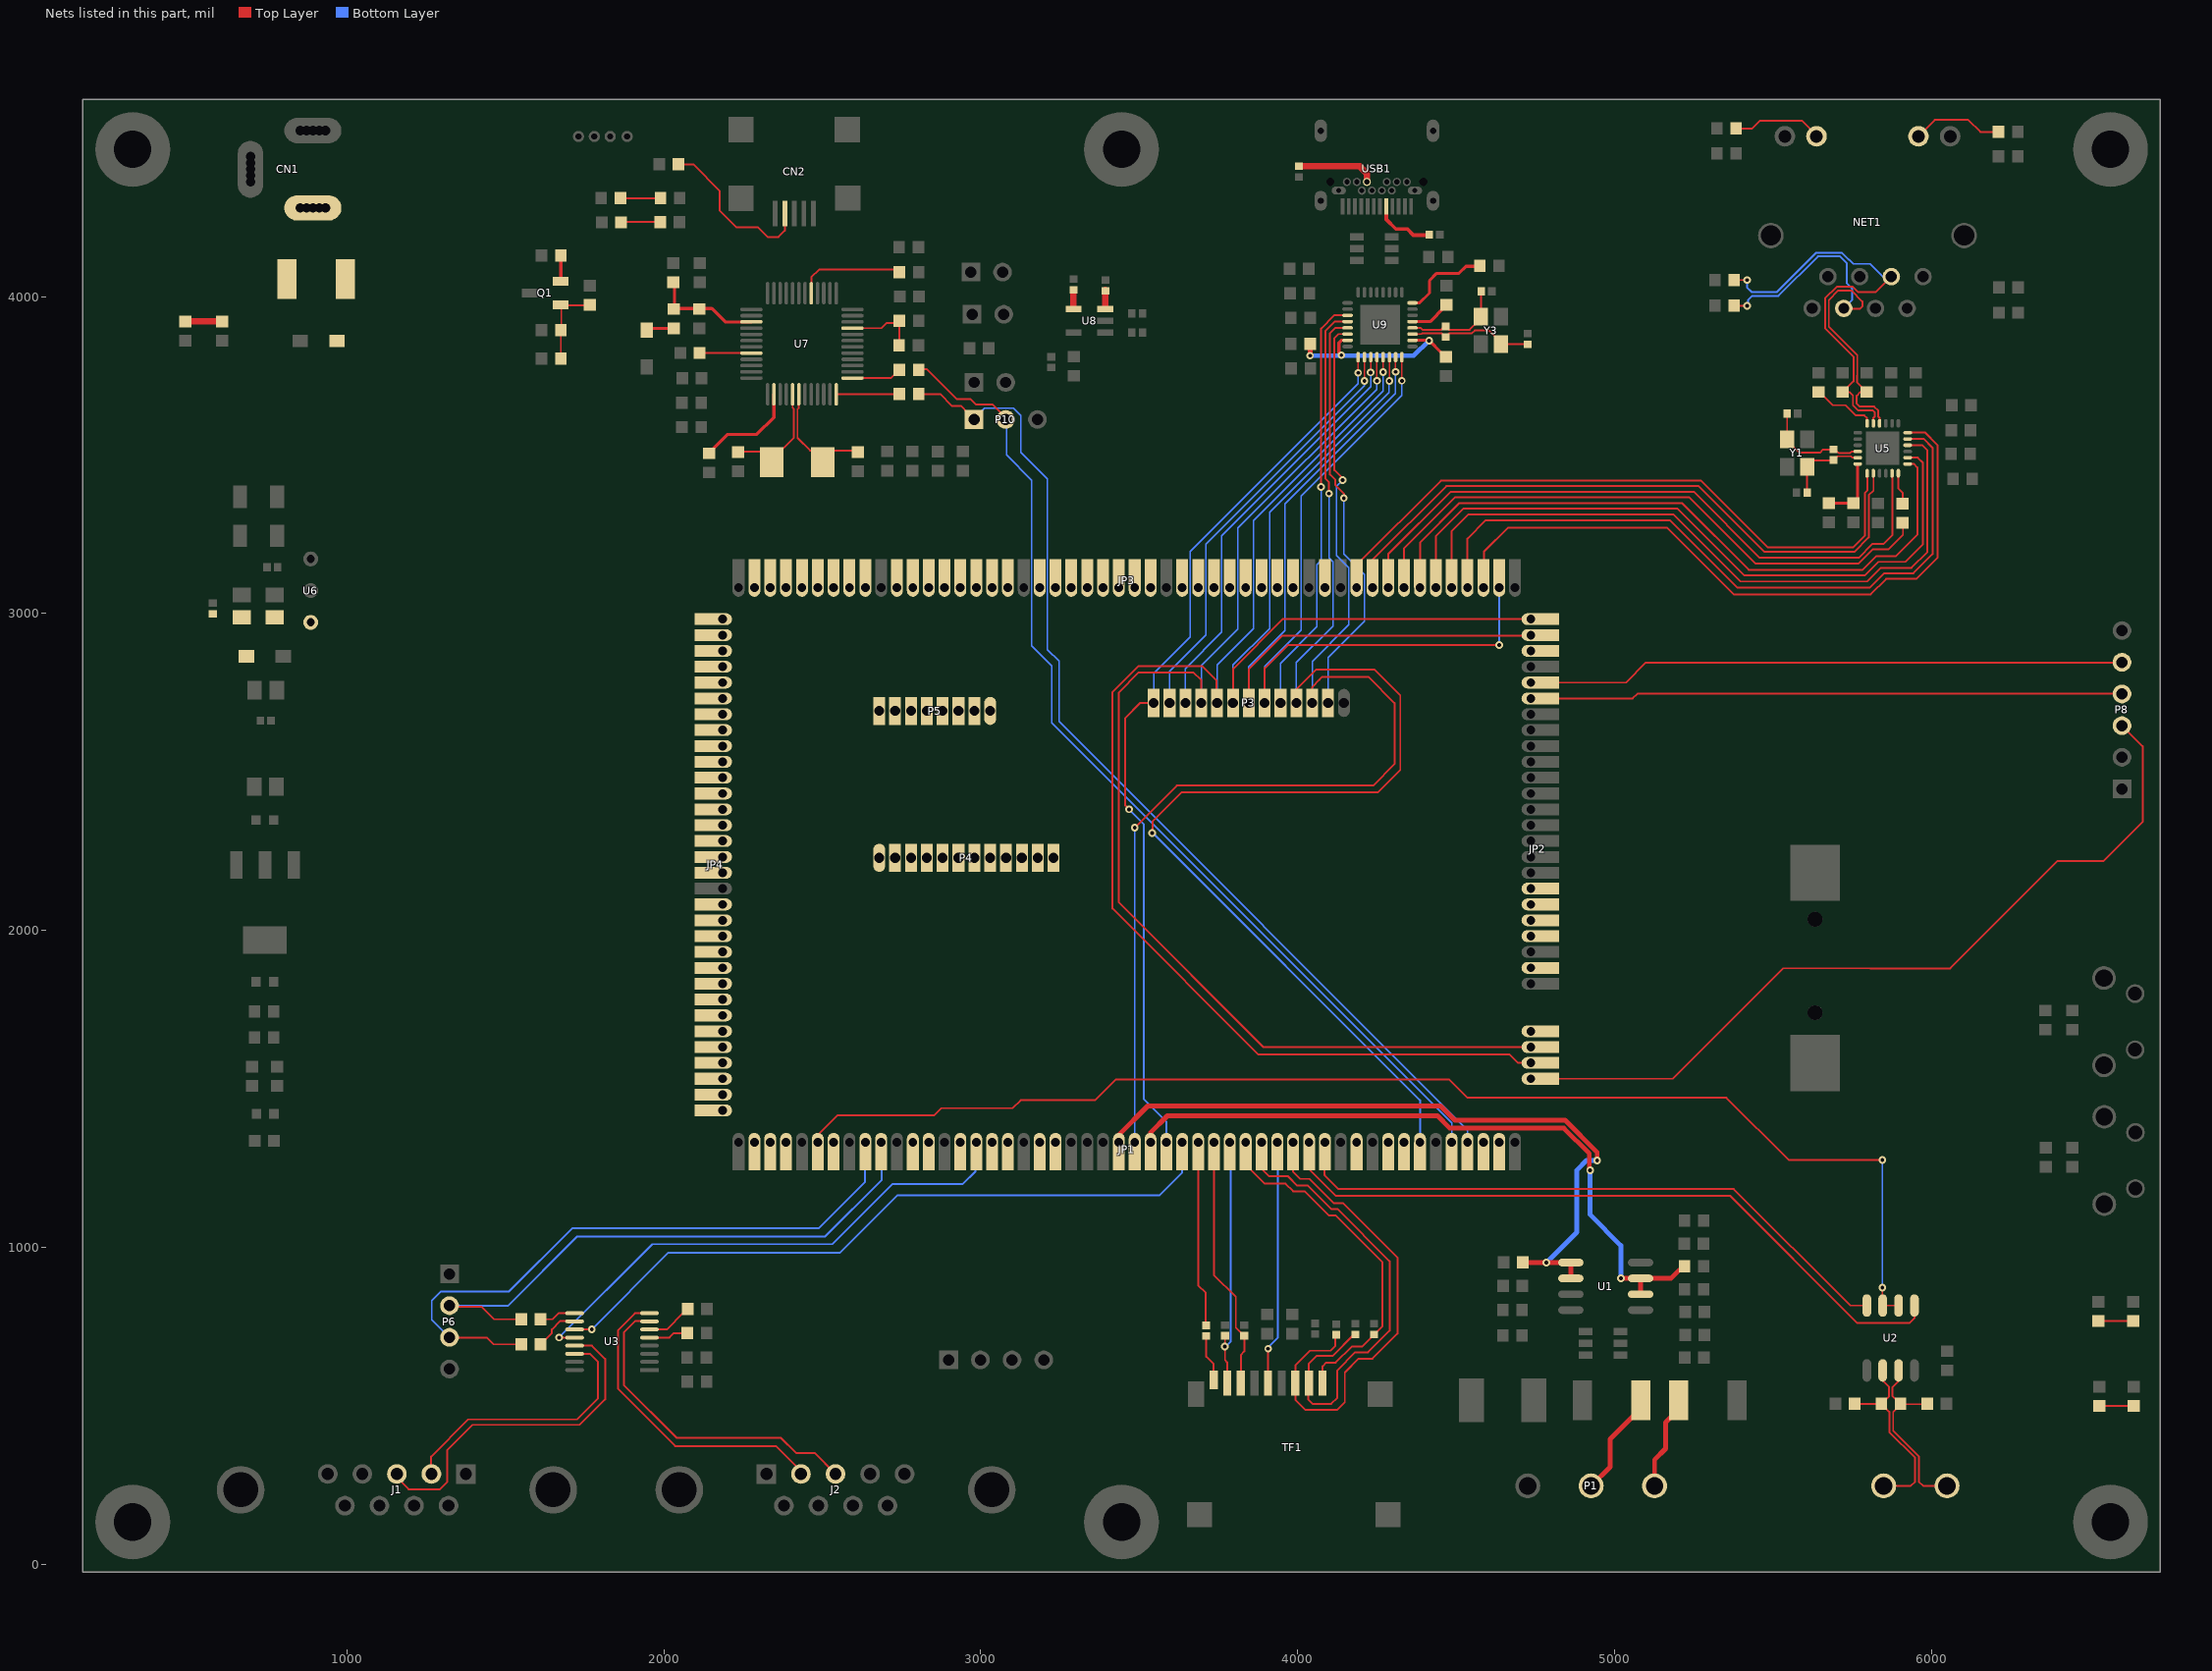
[diagram p0: the nets of this part, all layers, seen from the top]
# Altium PCB MISC105202-15.PcbDoc (part 3 of 4)
Units mil, origin at the board's own origin, x right, y up, seen from the top; angles counter-clockwise.
Board outline 6555.12 x 4645.67 mil, 2 copper layers (Top Layer, Bottom Layer); 182 components, 258 nets, 994 pads, 145 vias.
Unrouted connection lines stored in the file: 1.

## Via types
v1: diameter 24, hole 12, Top Layer to Bottom Layer, 128 vias
v2: diameter 19.68, hole 7.87, Top Layer to Bottom Layer, 9 vias
v3: diameter 50, hole 50, Top Layer to Bottom Layer, 4 vias
v4: diameter 30, hole 15, Top Layer to Bottom Layer, 2 vias
v5: diameter 137.8, hole 137.8, Top Layer to Bottom Layer, 2 vias

## Nets (pads, with @x,y where several pads share a name; then routed paths per layer and width w, separated by ;. In a path a pad name is that pad's centre, name@x,y a point inside that pad or via, vN(x,y) a via of type N, cw(c..) or ccw(c..) an arc to the next point about the centre after c; other vN are vias at no path point) (continued)
NetC9_2: C9.2 U3.5 | length 119.6
  Top Layer w6: U3.5@1955,715.36 2018.36,715.36 2032,729 C9.2@2069,729
NetC11_2: C11.2 U3.6 | length 130
  Top Layer w6: U3.6@1955,740.95 2009.95,740.95 C11.2@2063,794
NetC25_2: C25.2 C26.2 U5.6 | length 202.7
  Top Layer w10: C25.2@5676,3348.31 C26.2@5754,3348.31 C26.2@5754.32,3348.31 ; C26.2@5766,3346 5767,3347 5767,3393 5767,3399 U5.6@5767,3470
NetC27_1: C27.1 R32.2 U5.4 Y1.1 | length 314.9
  Top Layer w6: C27.1@5544.5,3624.5 Y1.1@5544.5,3549.31 5544.5,3545.5 5583,3507 5648,3507 5658,3517 R32.2@5688,3517 ; R32.2@5700,3513 5707,3506 5743,3506 5748.16,3511.16 U5.4@5767.26,3511.16
NetC29_1: C29.1 R32.1 U5.5 Y1.3 | length 214
  Top Layer w6: C29.1@5607.73,3381 Y1.3@5607.73,3452.73 ; Y1.3@5620,3483 5689.73,3483 R32.1@5691,3484.27 ; R32.1@5700,3492 5704,3496 5746,3496 5750.53,3491.47 U5.5@5767.26,3491.47
NetC31_2: C31.2 C32.2 C33.1 D7.1 U6.3
NetC57_2: C57.2 U8.4 | length 60.3
  Top Layer w20: U8.4@3293,3961 3293,3969 C57.2@3293,4021.27
NetC63_1: C63.1 R60.2 U9.27 Y3.3 | length 357.8
  Top Layer w6: U9.27@4362.36,3881.47 4390.47,3881.47 4393,3884 4454,3884 R60.2@4461,3877 ; R60.2@4467,3872.27 4478.73,3884 4550,3884 4559,3893 4604,3893 Y3.3@4628,3869 ; Y3.3@4650.27,3849.27 C63.1@4726,3849.27
NetC64_1: C64.1 R60.1 U9.28 Y3.1 | length 305
  Top Layer w6: U9.28@4362.36,3901.16 4387.84,3901.16 4394,3895 4453,3895 R60.1@4461,3903 ; R60.1@4467,3905.73 4477.73,3895 4543,3895 Y3.1@4570,3922 ; C64.1@4578,4018 4578.5,4017.5 Y3.1@4578.5,3936.31
NetC65_2: C65.2 U9.29 | length 117.9
  Top Layer w10: U9.29@4362.36,3920.84 4417.84,3920.84 C65.2@4462,3965
NetC66_2: C66.2 C67.2 U9.15 U9.26 | length 606.2
  Top Layer w4: C67.2@4044,3852 C67.2@4044.21,3851.79
  Top Layer w10: v1(4039.31,3813.31) v1@4039.31,3819.69 ; v1@4130,3823 4130,3854 4137.79,3861.79 U9.15@4157.64,3861.79 ; U9.26@4362.36,3861.79 4414.21,3861.79 v1(4415,3861) C66.2@4454,3822
  Top Layer w15: C67.2@4039.31,3851 4039.31,3819.69 v1@4041,3818
  Bottom Layer w15: v1(4039.31,3813.31) 4366.31,3813.31 v1@4415,3862
  other v1: 4138,3815
NetCN1_1: CN1.1 F2.2
NetCN2_4: CN2.4 R52.2 | length 499.1
  Top Layer w6: R52.2@2046.32,4417 2093,4417 2177,4333 2177,4271 2229,4219 2297,4219 2328,4188 2362,4188 2382,4208 CN2.4@2382,4232
NetD4_K: D4.K R18.1 | length 107.3
  Top Layer w6: R18.1@6527,767.69 6527.69,767 D4.K@6634,767
NetD5_K: D5.K R20.1 | length 103.1
  Top Layer w6: R20.1@6529,499.69 6628.31,499.69 D5.K@6631,497
NetD6_1: D6.1 F2.1
NetD9_A: D9.A R33.2 | length 115.3
  Top Layer w20: D9.A@491.68,3921.32 R33.2@607,3921.32
NetD12_2: D12.2 R34.1 | length 85.1
  Top Layer w10: D12.2@1946,3900 1946.31,3899.69 R34.1@2031,3899.69
NetD13_A: D13.A R50.2 | length 112.7
  Top Layer w6: D13.A@1877,4310 R50.2@1989.68,4310
NetD14_K: D14.K R51.2 | length 112.1
  Top Layer w6: D14.K@1877,4234 1878,4235 R51.2@1988.68,4235
NetF1_1: F1.1 P1.2 | length 289.9
  Top Layer w15: P1.2@4926,247.37 4986,307.37 4986,395 F1.1@5069,478
NetF3_1: F3.1 P1.1 | length 251.9
  Top Layer w15: P1.1@5126,247.37 5126,330 5161,365 5161,448 F3.1@5187,474
NetNET1_10: NET1.10 R26.1 | length 287.2
  Top Layer w6: NET1.10@5958.83,4505.54 6010.28,4557 6116,4557 6154,4519 R26.1@6209,4519
NetNET1_11: NET1.11 R25.1 | length 269
  Top Layer w6: R25.1@5383.31,4530 5434,4530 5459,4555 5591,4555 NET1.11@5627,4519
NetQ1_1: Q1.1 R54.1 R55.1 R56.2 | length 258.7
  Top Layer w6: R54.1@1675.31,3804 1675.31,3897.69 1677,3899.37 1677,3972 R55.1@1767,3972
NetQ1_2: Q1.2 R53.2 | length 84.6
  Top Layer w10: Q1.2@1675.21,4048.4 1675.21,4126.21 R53.2@1680,4131
NetR8_2: R8.2 U3.10 | length 135.6
  Top Layer w6: R8.2@1611.32,694 1647,729.68 1647,741 1673,767 U3.10@1710,767
NetR9_2: R9.2 U3.9 | length 115.4
  Top Layer w6: R9.2@1611.32,773 1649,773 1668.13,792.13 U3.9@1718.78,792.13
NetR16_2: R16.2 TF1.9 | length 142
  Top Layer w6: R16.2@3712,714 3712,655 3735.19,631.81 TF1.9@3735.19,581.56
NetR27_1: R27.1 U5.24 | length 183.2
  Top Layer w6: R27.1@5659,3686 5688,3657 5729,3657 5761,3625 5788,3625 5796.79,3616.21 U5.24@5796.79,3599.74
NetR29_2: R29.2 U5.12 | length 101.7
  Top Layer w6: U5.12@5895.21,3442.26 5895.21,3394.79 5909,3381 R29.2@5909,3346.32
NetR34_2: R34.2 R35.1 R38.2 U7.39 | length 343.9
  Top Layer w6: R38.2@2030,4036 R38.2@2030,4040
  Top Layer w10: R38.2@2027,4039 2030,4036 2034,4032 2034,3962 2152,3962 2194.1,3919.9 U7.39@2276.55,3919.9
NetR39_2: R39.2 U7.44 | length 159.2
  Top Layer w6: R39.2@2118,3820 2119.47,3821.47 U7.44@2276.55,3821.47
NetR40_2: R40.2 U7.2 | length 307.9
  Top Layer w6: R40.2@2155,3517 R40.2@2156.5,3518.5
  Top Layer w10: R40.2@2156,3519 2202,3565 2294,3565 2347.42,3618.42 U7.2@2347.42,3691.55
NetR42_1: R42.1 U7.29 | length 335.2
  Top Layer w6: U7.29@2465.53,4010.45 2465.53,4060.53 2490,4085 2732,4085 R42.1@2738,4079
NetR46_2: R46.2 U7.12 | length 201.3
  Top Layer w6: U7.12@2544.27,3691.55 2743.55,3691.55 R46.2@2745,3693
NetR47_2: R47.2 U7.13 | length 141.9
  Top Layer w6: U7.13@2595.45,3742.73 2715.73,3742.73 R47.2@2731,3758
NetR48_1: R48.1 R49.2 U7.21 | length 222
  Top Layer w6: U7.21@2595.45,3900.21 2687.21,3900.21 2704,3917 R48.1@2746,3917 ; R49.2@2742.68,3846 2742.68,3908.68 R48.1@2744,3910
NetR57_1: R57.1 U8.3 | length 55.1
  Top Layer w20: U8.3@3393,3966 3393.27,3966.27 R57.1@3393.27,4021
NetR58_1: R58.1 USB1.B5 | length 249
  Top Layer w20: R58.1@4004,4410.73 4196.27,4410.73 4218,4389 USB1.B5@4218,4363
NetR59_2: R59.2 USB1.A5 | length 195.4
  Top Layer w12: USB1.A5@4279.53,4284.95 4279.53,4243.47 4310,4213 4346,4213 4365,4194 R59.2@4413,4194
NetR61_2: R61.2 U9.32 | length 283.2
  Top Layer w10: U9.32@4362.36,3979.9 4384.9,3979.9 4416,4011 4416,4050 4439,4073 4509,4073 4531,4095 R61.2@4575,4095
OSC_IN: C51.1 U7.5 Y2.2 | length 316.7
  Top Layer w6: C51.1@2251,3511 2367,3511 2411,3555 2411,3644 2406.47,3648.53 U7.5@2406.47,3691.55
OSC_OUT: C50.1 U7.6 Y2.1 | length 357.8
  Top Layer w6: U7.6@2426.16,3691.55 2426.16,3648.16 2422,3644 2422,3554 2462,3514 C50.1@2624,3514
PA1_RMII_REF_CLK: JP3.45 U5.14 | length 2107.9
  Top Layer w6: JP3.45@4436,3148 4436,3243 4524,3331 5198,3331 5409,3120 5789,3120 5832,3163 5917,3163 5973,3219 5973,3475 5956.53,3491.47 U5.14@5924.74,3491.47
PA2_ETH_MDIO: JP3.43 R29.1 | length 1873.2
  Top Layer w6: JP3.43@4336,3126.36 4336,3206 4496,3366 5236,3366 5445,3157 5769,3157 5815,3203 5865,3203 5910,3248 R29.1@5910,3277
PA3_ULPI_D0: JP3.49 P3.6 U9.24 | length 2333.4
  Top Layer w4: v1(4328.9,3734.1) U9.24@4328.9,3808.64
  Top Layer w6: P3.6@3896,2717.62 3896,2827 3969,2900 v1(4636,2900)
  Bottom Layer w4: P3.6@3896,2717.62 3896,2833 4011,2948 4011,3277 ; 4011,3280 4011,3277 ; v1@4329,3734 4329,3688 4011,3370 4011,3277
  Bottom Layer w6: v1(4636,2900) 4636,3065 JP3.49@4647,3076
PA4_ADC1_CH18: C1.2 JP1.25 U1.1 U1.2 | length 2263.7
  Top Layer w6: JP1.25@3436,1331.87 JP1.25@3436,1337 ; C1.2@4717,951 C1.2@4718,952
  Top Layer w15: JP1.25@3437,1337 3437,1356 3527,1446 4451,1446 4496,1401 4844,1401 4945,1300 v1(4945,1274) ; C1.2@4709,952 4718,952 v1(4785,952) 4856,952 4862,946 U1.2@4862,902
  Bottom Layer w15: v1(4785,952) v1@4785,955 ; v1@4788,955 4881,1048 4881,1205 4881,1244 4911,1274 v1(4945,1274)
PA5_ULPI_CK: JP1.26 P3.3 U9.14 | length 3728.2
  Top Layer w6: v1(3486,2324) 3619,2457 4238,2457 4306,2525 4306,2717 4223,2800 4078,2800 4068.5,2790.5 4046,2768 P3.3@4046,2717.62 ; v1@4142,3418 v1(4142,3421) 4142,3426 4116,3452 4116,3869 4128.47,3881.47 U9.14@4157.64,3881.47
  Bottom Layer w4: P3.3@4046,2717.62 4046,2849 4161,2964 4161,3145 4123,3183 4123,3401 v1@4141,3419
  Bottom Layer w6: JP1.26@3486,1331.87 3486,2079 ; 3486,2083 3486,2079 ; v1@3486,2322 3486,2079
PA6_ADC2_CH3: C5.2 JP1.27 U1.6 U1.7 | length 2167.1
  Top Layer w6: v1(4923,1243) v1@4923,1249
  Top Layer w15: JP1.27@3536,1331.87 3536,1362 3589,1415 4441,1415 4480,1376 4840,1376 4920,1296 v1@4920,1249 ; v1@5023,902 U1.7@5082,902 ; U1.6@5083,856 5082,857 U1.7@5082,902 ; C5.2@5213,929 5205,929 5178,902 U1.7@5082,902
  Bottom Layer w15: v1(4923,1243) 4923,1103 5020,1006 v1(5020,902)
PA7_CRS_DV: JP3.42 U5.11 | length 2038.8
  Top Layer w6: JP3.42@4286,3126.36 4286,3187 4483,3384 5250,3384 5458,3176 5770,3176 5813,3219 5848,3219 5876,3247 U5.11@5876,3438
PA8_MCO: JP2.30
PA9_U1T: JP1.46 P10.2 R47.1 | length 3181.2
  Top Layer w6: R47.1@2805,3771 2830,3771 2924,3677 2967,3677 2985,3659 3038,3659 P10.2@3071,3626
  Bottom Layer w4: P10.2@3081,3605 3081,3500 3160.7,3420.3 3160.7,2898.3 3224,2835 3224,2655 3838.5,2040.5 4486,1393 JP1.46@4486,1331.87
PA10_U1R: JP1.47 P10.1 R46.1 | length 3198.3
  Top Layer w6: R46.1@2804.31,3692 R46.1@2806.66,3689.66 ; R46.1@2809,3692 2872,3692 2909,3655 2937,3655 P10.1@2961,3631
  Bottom Layer w4: P10.1@3000,3635 3012.53,3647.53 3103.47,3647.53 3127,3624 3127,3508 3210.7,3424.3 3210.7,2886.3 3247,2850 3247,2659 4536,1370 JP1.47@4536,1331.87
PA11_USB1_FS_DM: JP1.48
PA12_USB1_FS_DP: JP1.49
PB0_ULPI_D1: JP2.31 P3.7 U9.23 | length 2313.9
  Top Layer w4: v1(4309.21,3762.21) U9.23@4309.21,3808.64
  Top Layer w6: P3.7@3846,2717.62 3846,2824 3952,2930 JP2.31@4733,2930
  Bottom Layer w4: P3.7@3846,2717.62 3846,2831 3960.7,2945.7 3960.7,3345.7 4309,3694 v1@4309,3756
PB1_ULPI_D2: JP2.32 P3.8 U9.22 | length 2386.3
  Top Layer w4: v1(4289.53,3733.47) U9.22@4289.53,3808.64
  Top Layer w6: P3.8@3797,2735 3797,2826 3952.87,2981.87 JP2.32@4736,2981.87
  Bottom Layer w4: P3.8@3796,2717.62 3796,2837 3911.3,2952.3 3911.3,3319.3 4289,3697 v1@4289,3730
PB2_QSPI_CLK: JP1.12
PB3_SDIO2_D2: JP1.10 P6.2 R9.1 | length 1872.3
  Top Layer w6: P6.2@1336,813 1425,813 1465,773 R9.1@1550.69,773
  Bottom Layer w6: P6.2@1324,816 1509,816 1727,1034 2509,1034 2687,1212 JP1.10@2687,1326
PB4_SDIO2_D3: JP1.9 P6.3 R8.1 | length 1997.9
  Top Layer w6: P6.3@1339,715 1442,715 1463,694 R8.1@1550.69,694
  Bottom Layer w6: P6.3@1324,716 1268,772 1268,832 1297,861 1512,861 1711,1060 2488,1060 2635,1207 JP1.9@2635,1323
PB5_ULPI_D7: JP1.28 P3.13 U9.17 | length 2861.3
  Top Layer w4: v1(4191.1,3759.1) U9.17@4191.1,3808.64
  Top Layer w6: v1(3468,2382) 3456,2394 3456,2670 3503.62,2717.62 P3.13@3546,2717.62
  Bottom Layer w4: P3.13@3546,2717.62 3546,2811 3661,2926 3661,3195 4191.1,3725.1 v1(4191.1,3759.1)
  Bottom Layer w6: v1@3467,2383 v1(3468,2382) 3515,2335 3515,1467 3586,1396 JP1.28@3586,1331.87
PB6_I2C1_SCL: JP3.2
PB7_I2C1_SDA: JP3.3
PB8_SDIO1_CKIN: JP1.37 U2.1 | length 2141.3
  Top Layer w6: JP1.37@4039,1250 4039,1244 4120,1163 5364,1163 5765,762 5931,762 5947,778 U2.1@5947,799
PB9_SDIO1_CDIR: JP1.38 U2.4 | length 1930.1
  Top Layer w6: 4085,1227 JP1.38@4085,1277 ; 4086,1227 4129,1184 5376,1184 5743.64,816.36 U2.4@5796,816.36
PB10_ULPI_D3: JP2.4 P3.9 U9.21 | length 4003.9
  Top Layer w4: P3.9@3746,2717.62 P3.9@3746,2744 ; v1(4269.84,3761.84) U9.21@4269.84,3808.64
  Top Layer w6: P3.9@3744,2744 3744,2788 3698,2834 3498,2834 3416,2752 3416,2069 3877,1608 4668.87,1608 4695,1581.87 JP2.4@4736,1581.87 JP2.4@4780.49,1581.87
  Bottom Layer w4: P3.9@3746,2717.62 3746,2838 3861,2953 3861,3293 4270,3702 v1@4270,3757
PB11_ULPI_D4: JP2.5 P3.10 U9.20 | length 3883.2
  Top Layer w4: P3.10@3696,2717.62 P3.10@3696,2735 ; v1(4250.16,3734.16) U9.20@4250.16,3808.64 ; JP2.5@4736,1631.87 JP2.5@4780.49,1631.87
  Top Layer w6: P3.10@3696,2735 3696,2789 3671,2814 3499,2814 3436,2751 3436,2723 3436,2521 3436,2518 3436,2088 3892.13,1631.87 JP2.5@4736,1631.87
  Bottom Layer w4: P3.10@3696,2717.62 3696,2836 3811,2951 3811,3269 4249,3707 v1@4249,3733
PB12_ULPI_D5: P3.11 U9.19 | length 1333.1
  Top Layer w4: v1(4230.47,3760.47) U9.19@4230.47,3808.64
  Bottom Layer w4: P3.11@3646,2717.62 3646,2826 3760.7,2940.7 3760.7,3245.7 4230.47,3715.47 v1(4230.47,3760.47)
PB13_ULPI_D6: P3.12 U9.18 | length 1345.7
  Top Layer w4: v1(4210.79,3733.79) U9.18@4210.79,3808.64
  Bottom Layer w4: P3.12@3596,2717.62 3596,2817 3711,2932 3711,3219 4210.79,3718.79 v1(4210.79,3733.79)
PB14_SDIO2_D0: JP1.6 U2.2 U2.3 | length 4085
  Top Layer w6: JP1.6@2484,1352 2549,1417 2854,1417 2876,1439 3101,1439 3126,1464 3361,1464 3427,1530 4478,1530 4536,1472 5353,1472 5549,1276 v1(5845,1276) ; JP1.6@2486,1287.38 JP1.6@2486,1331.87 JP1.6@2486,1341 ; U2.3@5842,838 5845,841 v1(5845,873) ; U2.3@5844,816 5844.36,816.36 U2.3@5846,816.36 U2.2@5896,816.36
  Bottom Layer w6: v1(5845,873) v1(5845,1276)
PC0_ULPI_STP: P3.2 U9.13 | length 1320.9
  Top Layer w6: v1(4146,3364) 4146,3378 4119,3405 4119,3421 4102,3438 4102,3884 4119.16,3901.16 U9.13@4157.64,3901.16
  Bottom Layer w4: P3.2@4096,2717.62 4096,2861 4211,2976 4211,3123 4146,3188 v1@4146,3363
PC1_ETH_MDC: JP3.44 U5.13 | length 2094.1
  Top Layer w6: JP3.44@4386,3126.36 4386,3224 4510,3348 5213,3348 5423,3138 5783,3138 5826,3181 5888,3181 5955,3248 5955,3461 5944,3472 U5.13@5929,3472
PC2_C: JP1.43
PC2_DFSDM_CLK: JP2.27 P8.4 | length 1825.8
  Top Layer w6: JP2.27@4780.49,2731.87 5056.87,2731.87 5072,2747 P8.4@6600,2747
PC3_C: JP1.42
PC3_DFSDM_DATA1: JP2.28 P8.5 | length 1841.7
  Top Layer w6: JP2.28@4780.49,2781.87 5035.87,2781.87 5099,2845 P8.5@6596,2845
PC4_RMII_RXD0: JP3.41 U5.8 | length 2012.6
  Top Layer w6: JP3.41@4236,3126.36 4236,3169 4469,3402 5265,3402 5473,3194 5756,3194 5802,3240 5802,3373 5817,3388 U5.8@5817,3436
PC5_RMII_RXD1: JP3.40 U5.7 | length 2035.9
  Top Layer w6: JP3.40@4186,3126.36 4186,3153 4452,3419 5273,3419 5484,3208 5752,3208 5790,3246 5790,3381 5797,3388 U5.7@5797,3435
PC6_SDIO1_D0DIR: JP1.29 U3.11 | length 2206.9
  Top Layer w6: U3.11@1718.78,740.95 v1(1772.95,740.95)
  Bottom Layer w6: v1(1772.95,740.95) 2015,983 2556,983 2737,1164 3564,1164 3578.5,1178.5 3635,1235 JP1.29@3635,1321
PC7_SDIO1_ACT: JP1.30 R16.1 | length 542.3
  Top Layer w6: JP1.30@3686,1287.38 3686,880 3710,856 R16.1@3710,755
PC8_SDIO1_D0: JP1.31 R12.1 TF1.7 | length 778.8
  Top Layer w6: JP1.31@3736,1307 3736,913 3805,844 3805,746.23 3829.96,721.27 R12.1@3831,721.27 ; TF1.7@3820.69,571.56 3820.69,660.69 3832,672 R12.1@3832,720
PC9_SDIO1_D1: JP1.32 R13.1 TF1.8 | length 793.1
  Top Layer w6: R13.1@3771,720 3771,709 3771,686 3771,685 3771,644 3777.69,637.31 TF1.8@3777.69,571.56
  Bottom Layer w6: v1(3770,687) 3770,686 3771,685 3789,703 JP1.32@3789,1317
PC10_SDIO1_D2: JP1.33 R11.1 TF1.1 | length 1043.5
  Top Layer w6: JP1.33@3843,1253 3850,1246 3851,1246 3896,1201 3962,1201 3986,1177 4022,1177 4098,1101 4120,1101 4267,954 4267,750.23 4242.04,725.27 R11.1@4241,725.27 ; TF1.1@4078.69,571.56 4078.69,624.69 4090,636 4120,636 4171,687 4203,687 R11.1@4240,724
PC11_SDIO1_D3: JP1.34 R14.1 TF1.2 | length 1457.2
  Top Layer w6: JP1.34@3886,1287.38 3886,1249 3911,1224 3970,1224 3999,1195 4032,1195 4106,1121 4125,1121 4290,956 4290,737 4222,669 4182,669 4125,612 4125,525 4106,506 4047,506 4034,519 TF1.2@4034,546 ; TF1.2@4035.69,571.56 4035.69,633.69 4060,658 4111,658 R14.1@4176,723
PC12_SDIO1_CK: JP1.35 TF1.5 | length 758.6
  Top Layer w6: TF1.5@3906.69,571.56 3906.69,644.69 ; 3907,645 v1(3907,680)
  Bottom Layer w6: v1@3908,685 3938,715 JP1.35@3938,1323
PC13_TAMP: JP3.38
PD0_FMC_D2: JP4.12
PD1_FMC_D3: JP4.11
PD2_SDIO1_CMD: JP1.36 R15.1 TF1.3 | length 1492.9
  Top Layer w6: JP1.36@3984,1256 JP1.36@3984,1264 ; JP1.36@3986,1256 3986,1238 4008,1216 4038,1216 4115,1139 4144,1139 4315,968 4315,728 4236,649 4193,649 4149,605 4149,512 4124,487 4025,487 3992.69,519.31 TF1.3@3992.69,571.56 3992.69,627.69 4039,674 4104,674 4119,689 R15.1@4119,725
PD3: JP2.3 P8.3 | length 2552
  Top Layer w4: JP2.3@4780.49,1531.87 5183.87,1531.87 5532,1880 5807,1880
  Top Layer w6: 5807,1880 6059,1880 6398,2219 6543,2219 6666,2342 6666,2581 P8.3@6601,2646
PD4_FMC_NOE: JP4.2
PD5_FMC_NWE: JP4.1
PD6_FMC_NWAIT: JP1.7
PD7_FMC_NE1: P4.9
PD8_FMC_D13: JP4.30
PD9_FMC_D14: JP4.31
PD10_FMC_D15: JP4.32
PD11_FMC_A16: JP1.2
PD12_FMC_A17: JP1.3
PD13_FMC_A18: JP1.4
PD14_FMC_D0: JP4.14
PD15_FMC_D1: JP4.13
PE2_FMC_A23: JP2.10
PE3_FMC_A19: JP2.12
PE4_FMC_A20: JP2.13
PE5_FMC_A21: JP2.14
PE6_FMC_A22: JP2.15
PE7_FMC_D4: JP4.10
PE8_FMC_D5: JP4.9
PE9_FMC_D6: JP4.8
PE10_FMC_D7: JP4.7
PE11_FMC_D8: JP4.25
PE12_FMC_D9: JP4.26
PE13_FMC_D10: JP4.27
PE14_FMC_D11: JP4.28
PE15_FMC_D12: JP4.29
PF0_FMC_A0: JP4.6
PF1_FMC_A1: JP4.5
PF2_FMC_A2: JP4.4
PF3_FMC_A3: JP4.3
PF4_FMC_A4: JP4.16
PF5_FMC_A5: JP4.17
PF6_QSPI_BK1_IO3: JP1.20
PF7_QSPI_BK1_IO2: JP1.15
PF8_QSPI_BK1_IO0: JP1.13
PF9_QSPI_BK1_IO1: JP1.18
PF10_LCD_BL_CTRL: JP3.5
PF12_FMC_A6: JP4.18
PF13_FMC_A7: JP4.19
PF14_FMC_A8: JP4.20
PF15_FMC_A9: JP4.21
PG0_FMC_A10: JP4.22
PG1_FMC_A11: JP4.23
PG2_FMC_A12: JP4.24
PG3_FMC_A13: P4.10
PG4_FMC_A14: P4.11
PG5_FMC_A15: P4.12
PG6_QSPI_BK1_NCS: JP1.17
PG7_SAI1_MCLK_A: JP2.6
PG9_QSPI_BK2_IO2: JP1.16 U3.12 | length 1666.8
  Top Layer w6: v1(1669.64,715.36) U3.12@1718.78,715.36
  Bottom Layer w6: v1(1669.64,715.36) 1964.28,1010 2532,1010 2722,1200 2944,1200 2984,1240 JP1.16@2984,1326
PG10_LED: JP1.40
PG11_RMII_TX_EN: JP3.46 U5.16 | length 2165.6
  Top Layer w6: JP3.46@4486,3126.36 4486,3260 4539,3313 5185,3313 5397,3101 5797,3101 5840,3144 5937,3144 5987,3194 5987,3515 5971,3531 U5.16@5932,3531
PG12_RMII_TXD1: JP3.48 U5.18 | length 2132.1
  Top Layer w6: JP3.48@4586,3126.36 JP3.48@4586,3152 ; JP3.48@4588,3152 4588,3195 4664,3271 5165,3271 5376,3060 5808,3060 5857,3109 5952,3109 6019,3176 6019,3531 5979,3571 U5.18@5925,3571
PG13_RMII_TXD0: JP3.47 U5.17 | length 2155.6
  Top Layer w6: JP3.47@4536,3126.36 4536,3236 4594,3294 5175,3294 5387,3082 5806,3082 5851,3127 5943,3127 6003,3187 6003,3523 5975,3551 U5.17@5927,3551
PG14_QSPI_BK2_IO3: JP1.21
PH4_ULPI_NXT: P3.5 U9.11 | length 1337.7
  Top Layer w6: v1(4074,3399) 4074,3469 ; 4074,3464 4074,3469 ; U9.11@4157.64,3940.53 4115.53,3940.53 4074,3899 4074,3469
  Bottom Layer w4: P3.5@3946,2717.62 3946,2843 4061,2958 4061,3154 4075,3168 v1@4075,3396
PH8_FMC_D16: P4.1
PH9_FMC_D17: P4.2
PH10_FMC_D18: P4.3
PH11_FMC_D19: P4.4
PH12_FMC_D20: P4.5
PH13_FMC_D21: P4.6
PH14_FMC_D22: P4.7
PH15_FMC_D23: P4.8
PI0_FMC_D24: P5.1
PI1_FMC_D25: P5.2
PI2_FMC_D26: P5.3
PI3_FMC_D27: P5.4
PI6_FMC_D28: P5.5
PI7_FMC_D29: P5.6
PI8_TOUCH_INT: JP3.4
PI9_FMC_D30: P5.7
PI10_FMC_D31: P5.8
PI11_ULPI_DIR: JP1.44 P3.4 U9.12 | length 4191.2
  Top Layer w6: v1@3542,2311 3542,2344 3634,2436 4254,2436 4324,2506 4324,2741 4242,2823 4059,2823 3996,2760 P3.4@3996,2717.62 ; v1(4099,3378) 4099,3414 4088,3425 4088,3892 4116.84,3920.84 U9.12@4157.64,3920.84
  Bottom Layer w4: P3.4@3996,2717.62 3996,2845 4111,2960 4111,3163 4099,3175 v1@4099,3375 ; v1@4098,3376 v1@4099,3375 ; v1(4099,3378) v1@4099,3375
  Bottom Layer w6: v1(3541,2307) 3541,2309 4386,1464 JP1.44@4386,1331.87
PI12_LCD_HSYNC: JP3.8
PI13_LCD_VSYNC: JP3.7
PI14_LCD_CLK: JP3.9
PI15_LCD_R0: JP3.36
PJ0_LCD_R1: JP3.35
PJ1_LCD_R2: JP3.34
PJ2_LCD_R3: JP3.33
PJ3_LCD_R4: JP3.32
PJ4_LCD_R5: JP3.31
PJ5_LCD_R6: JP3.30
PJ6_LCD_R7: JP3.29
PJ7_LCD_G0: JP3.27
PJ8_LCD_G1: JP3.26
PJ9_LCD_G2: JP3.25
PJ10_LCD_G3: JP3.24
PJ11_LCD_G4: JP3.23
PJ12_LCD_B0: JP3.18
PJ13_LCD_B1: JP3.17
PJ14_LCD_B2: JP3.16
PJ15_LCD_B3: JP3.15
PK0_LCD_G5: JP3.22
PK1_LCD_G6: JP3.21
PK2_LCD_G7: JP3.20
PK3_LCD_B4: JP3.14
PK4_LCD_B5: JP3.13
PK5_LCD_B6: JP3.12
PK6_LCD_B7: JP3.11
PK7_LCD_DE: JP3.6
RD_N: C21.1 NET1.6 R21.1 U5.22 | length 1316.1
  Top Layer w6: C21.1@5377.31,3971 v1(5418,3971) ; NET1.6@5732,3962 5775,3962 5782,3969 5782,3984 5747,4019 5706,4019 5676,3989 5676,3904.97 5766,3814.97 5766,3751 5765,3751 5765,3729.69 R21.1@5796,3698.69 5775.69,3698.69 5764,3687 5764,3662 5773,3653 5819.29,3653 5832.32,3639.97 5832.32,3620.84 5836.16,3617 U5.22@5836.16,3599.74
  Bottom Layer w6: v1@5421,3974 5421,3988 5435,4002 5517,4002 5641.55,4126.55 5711.55,4126.55 5732,4106.09 5732,4043 5749,4026 5749,3988.43 NET1.6@5723.2,3962.63
RD_P: C20.1 NET1.3 R22.1 U5.23 | length 1375.8
  Top Layer w6: C20.1@5377.31,4052 v1(5418,4052) ; 5752,3675 5752,3674 ; U5.23@5816.47,3599.74 5816.47,3617 5820.32,3620.84 5820.32,3635 5814.32,3641 5768.03,3641 5752,3657.03 5752,3674 ; NET1.3@5866,4057 5822.49,4013.49 5769.49,4013.49 5751.97,4031 5701.03,4031 5664,3993.97 5664,3900 5754,3810 5754,3732.69 R22.1@5720,3698.69 5741.31,3698.69 5752,3688 5752,3674
  Bottom Layer w6: v1@5418,4048 5418,4029 5433,4014 5512.03,4014 5636.58,4138.55 5716.52,4138.55 5738.53,4116.53 ; 5739,4117 5753,4103 5806,4103 5846.37,4062.63 NET1.3@5873.2,4062.63
RS232_IN-1: J1.3 U3.13 | length 1088.8
  Top Layer w6: J1.3@1159,273 1195,237 1294,237 1317,260 1317,361 1396,440 1735,440 1815,520 1815,648 1773.23,689.77 U3.13@1718.78,689.77
RS232_IN-2: J2.2 U3.8 | length 987
  Top Layer w6: U3.8@1955,792.13 1909.13,792.13 1856,739 1856,553 2036,373 2354,373 J2.2@2430,297
RS232_OUT-1: J1.2 U3.14 | length 843.3
  Top Layer w6: J1.2@1266,299 1266,340 1383,457 1726,457 1793,524 1793,638 1766.82,664.18 U3.14@1718.78,664.18
RS232_OUT-2: J2.3 U3.7 | length 1033.3
  Top Layer w6: U3.7@1943,767 1910,767 1874,731 1874,566 2041,399 2370,399 2418,351 2476,351 J2.3@2542,285
RS485_A: P2.1 R6.2 R7.2 U2.6 | length 558
  Top Layer w6: R7.2@5762,506 R6.2@5841.68,506 5866,530.32 5866,560 5846,580 U2.6@5846,588 ; P2.1@5849,247.37 5934.37,247.37 5948,261 5948,336 5867,417 5867,481 R6.2@5853,495
RS485_B: P2.2 R5.2 R6.1 U2.7 | length 571.4
  Top Layer w6: U2.7@5894,592 5894,576 5877,559 5877,530 5901,506 R6.1@5902.31,506 ; R5.2@5988,505 5903,505 5879,481 5879,421.97 5960,340.97 5960,261 5973.63,247.37 P2.2@6049,247.37